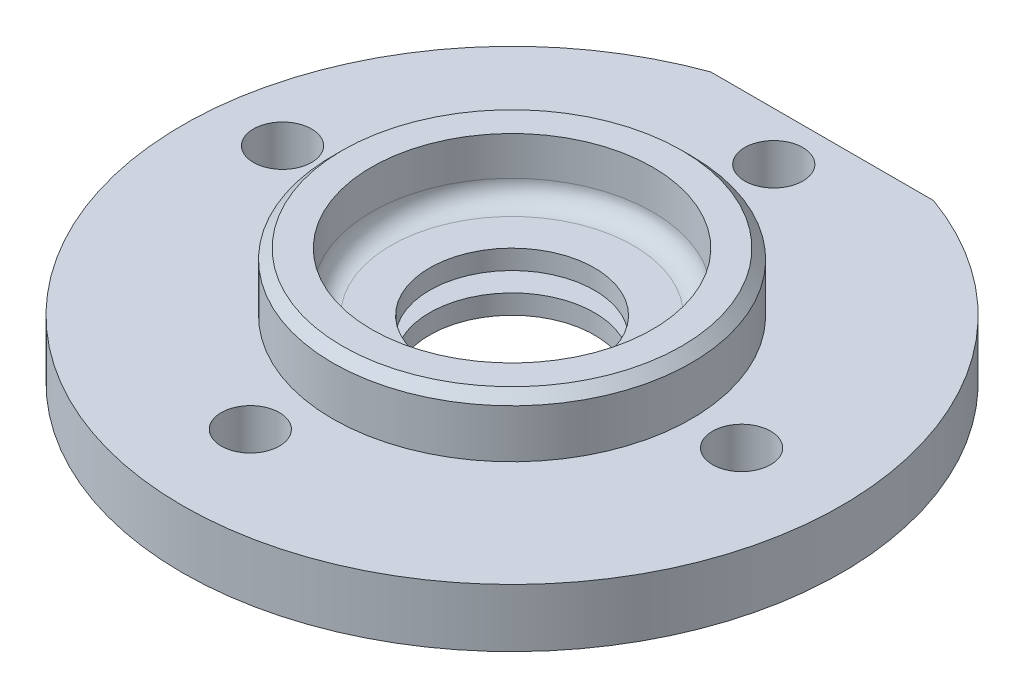
from build123d import *

# Parameters (mm, degrees)
SKETCH1_R           = 34
BOSS_EXTRUDE1_DEPTH = 6
SKETCH2_R           = 18.5
BOSS_EXTRUDE2_DEPTH = 6
SKETCH3_R           = 14.5
CUT_EXTRUDE1_DEPTH  = 6
SKETCH4_R           = 8.5
CUT_EXTRUDE2_DEPTH  = 2
SKETCH5_R           = 12.5
CUT_EXTRUDE3_DEPTH  = 2
SKETCH6_R           = 8.5
CUT_EXTRUDE4_DEPTH  = 2
CHAMFER1_SIZE       = 1
FILLET1_R           = 2
SKETCH7_W           = 39.246802542
SKETCH7_H           = 4
CUT_EXTRUDE5_DEPTH  = 23
SKETCH8_R           = 3
CUT_EXTRUDE6_DEPTH  = 80


with BuildPart() as part:
    # Sketch1 → Boss-Extrude1 (new body)
    with BuildSketch(Plane(origin=(0, 0, 0), x_dir=(1, 0, 0), z_dir=(0, 1, 0))):
        with Locations(Location((0, 0, 0), (0, 0, 270))):
            Circle(SKETCH1_R)
    extrude(amount=BOSS_EXTRUDE1_DEPTH)

    # Sketch2 → Boss-Extrude2 (add)
    with BuildSketch(Plane(origin=(0, 6, 0), x_dir=(1, 0, 0), z_dir=(0, 1, 0))):
        with Locations(Location((0, 0, 0), (0, 0, 270))):
            Circle(SKETCH2_R)
    extrude(amount=BOSS_EXTRUDE2_DEPTH)

    # Sketch3 → Cut-Extrude1 (cut)
    with BuildSketch(Plane(origin=(0, 12, 0), x_dir=(1, 0, 0), z_dir=(0, 1, 0))):
        with Locations(Location((0, 0, 0), (0, 0, 270))):
            Circle(SKETCH3_R)
    extrude(amount=-CUT_EXTRUDE1_DEPTH, mode=Mode.SUBTRACT)

    # Sketch4 → Cut-Extrude2 (cut)
    with BuildSketch(Plane(origin=(0, 6, 0), x_dir=(1, 0, 0), z_dir=(0, 1, 0))):
        with Locations(Location((0, 0, 0), (0, 0, 270))):
            Circle(SKETCH4_R)
    extrude(amount=-CUT_EXTRUDE2_DEPTH, mode=Mode.SUBTRACT)

    # Sketch5 → Cut-Extrude3 (cut)
    with BuildSketch(Plane(origin=(0, 4, 0), x_dir=(1, 0, 0), z_dir=(0, 1, 0))):
        with Locations(Location((0, 0, 0), (0, 0, 270))):
            Circle(SKETCH5_R)
    extrude(amount=-CUT_EXTRUDE3_DEPTH, mode=Mode.SUBTRACT)

    # Sketch6 → Cut-Extrude4 (cut)
    with BuildSketch(Plane(origin=(0, 2, 0), x_dir=(1, 0, 0), z_dir=(0, 1, 0))):
        with Locations(Location((0, 0, 0), (0, 0, 270))):
            Circle(SKETCH6_R)
    extrude(amount=-CUT_EXTRUDE4_DEPTH, mode=Mode.SUBTRACT)

    # Chamfer1
    chamfer1_edges = [part.edges().sort_by_distance(p)[0] for p in [
        (0, 12, -18.5),
    ]]
    chamfer(chamfer1_edges, length=CHAMFER1_SIZE)

    # Fillet1
    fillet1_edges = [part.edges().sort_by_distance(p)[0] for p in [
        (0, 6, -14.5),
    ]]
    fillet(fillet1_edges, radius=FILLET1_R)

    # Sketch7 → Cut-Extrude5 (cut)
    with BuildSketch(Plane(origin=(0, 6, 0), x_dir=(1, 0, 0), z_dir=(0, 1, 0))):
        with Locations((0, 34)):
            Rectangle(SKETCH7_W, SKETCH7_H)
    extrude(amount=-CUT_EXTRUDE5_DEPTH, mode=Mode.SUBTRACT)

    # Sketch8 → Cut-Extrude6 (cut)
    with BuildSketch(Plane(origin=(0, 6, 0), x_dir=(1, 0, 0), z_dir=(0, 1, 0))):
        with Locations(Location((0, 27, 0), (0, 0, 270))):
            Circle(SKETCH8_R)
        with Locations(Location((23.68, 0, 0), (0, 0, 270))):
            Circle(SKETCH8_R)
        with Locations(Location((-3.32, -23.68, 0), (0, 0, 270))):
            Circle(SKETCH8_R)
        with Locations(Location((-27, 3.32, 0), (0, 0, 270))):
            Circle(SKETCH8_R)
    extrude(amount=-CUT_EXTRUDE6_DEPTH, mode=Mode.SUBTRACT)


solid = part.part
